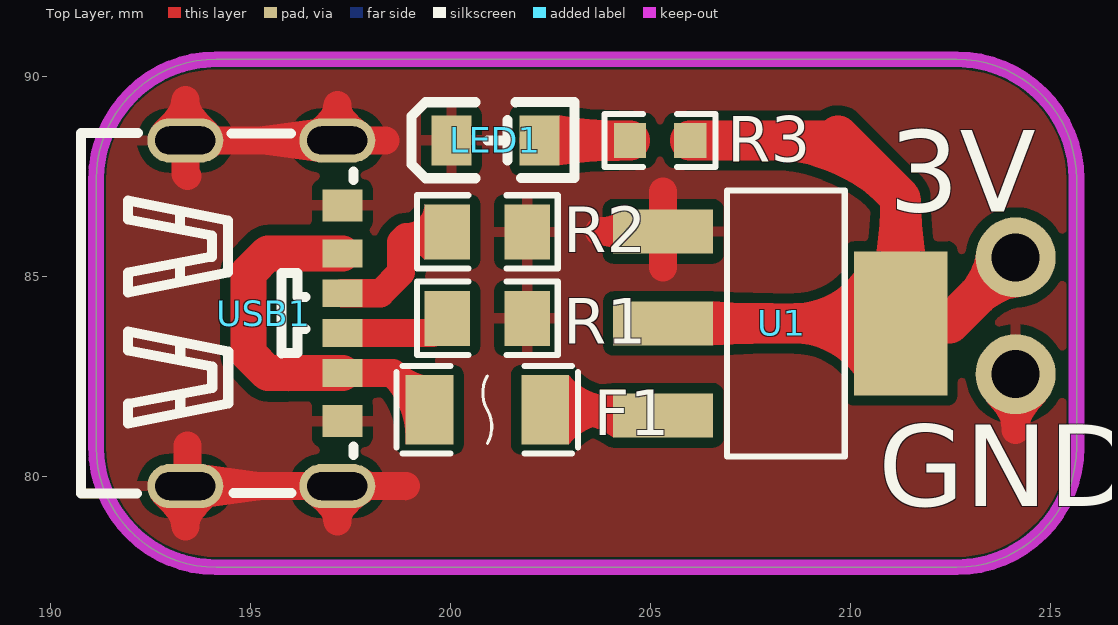
[diagram p0: Top Layer view]
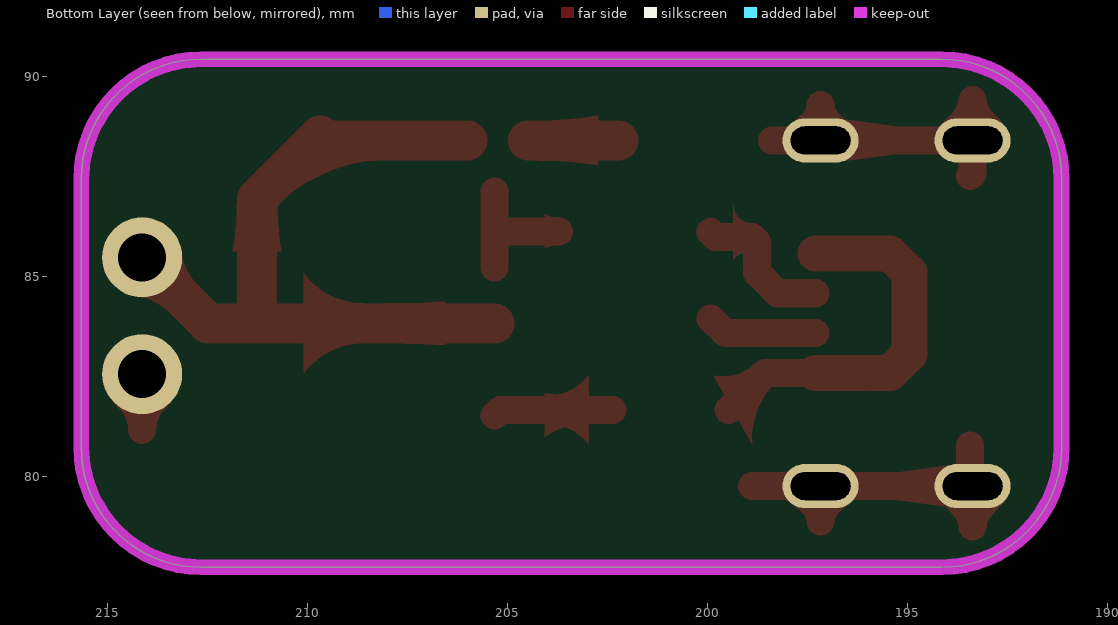
[diagram p1: Bottom Layer view, seen from below]
# Altium PCB MISC49884.pcbdoc
Units mm, origin at the board's own origin, x right, y up, seen from the top; angles counter-clockwise.
Board outline 24.51 x 12.7 mm, 2 copper layers (Top Layer, Bottom Layer), stack 1.58 mm thick; 7 components, 7 nets, 26 pads, 0 vias.

## Layer stack, top to bottom
Top Solder Mask Layer: solder mask 0.01, Dk 3.3
Top Layer: signal copper 0.035
Dielectric1: surface 1.51, FR4, Dk 4.5
Bottom Layer: signal copper 0.035
Bottom Solder Mask Layer: solder mask 0.01, Dk 3.3

## Board outline
194.135,90.424 ccw(c194.135,87.424) 191.135,87.424 191.135,80.724 ccw(c194.135,80.724) 194.135,77.724 212.646,77.724 ccw(c212.646,80.724) 215.646,80.724 215.646,87.424 ccw(c212.646,87.424) 212.646,90.424

## Design rules (kind name [scope] priority, off if disabled: settings)
BoardOutlineClearance copperThickness2oz_1 [All] p2 off: genericclearance=0.203 ignorepadtopadclearanceinfootprint=FALSE except(0: Arc-SplitContinuation Track-SplitContinuation SMDPad-SplitContinuation THPad-SplitContinuation Via-SplitContinuation Fill-SplitContinuation Region-SplitContinuation Poly-SplitContinuation Text-SplitContinuation Hole-SplitContinuation; 0.152: SMDPad-CutoutEdge THPad-CutoutEdge Via-CutoutEdge Fill-CutoutEdge Region-CutoutEdge Text-CutoutEdge Hole-CutoutEdge; 0.254: Poly-OutlineEdge Poly-CutoutEdge; 0.3: Arc-OutlineEdge Track-OutlineEdge SMDPad-OutlineEdge THPad-OutlineEdge Via-OutlineEdge Fill-OutlineEdge Region-OutlineEdge Text-OutlineEdge Hole-OutlineEdge Arc-CutoutEdge Track-CutoutEdge)
BoardOutlineClearance Plane_innerPlane_1 [All] p4 off: genericclearance=0.102 ignorepadtopadclearanceinfootprint=FALSE except(0: Arc-SplitContinuation Track-SplitContinuation SMDPad-SplitContinuation THPad-SplitContinuation Via-SplitContinuation Fill-SplitContinuation Region-SplitContinuation Poly-SplitContinuation Text-SplitContinuation Hole-SplitContinuation; 0.152: SMDPad-CutoutEdge THPad-CutoutEdge Via-CutoutEdge Fill-CutoutEdge Region-CutoutEdge Text-CutoutEdge Hole-CutoutEdge; 0.254: Poly-OutlineEdge Poly-CutoutEdge; 0.3: Arc-OutlineEdge Track-OutlineEdge SMDPad-OutlineEdge THPad-OutlineEdge Via-OutlineEdge Fill-OutlineEdge Region-OutlineEdge Text-OutlineEdge Hole-OutlineEdge Arc-CutoutEdge Track-CutoutEdge)
BoardOutlineClearance Copper_copperRegion_1 [All] p6 off: genericclearance=0.102 ignorepadtopadclearanceinfootprint=FALSE except(0: Arc-SplitContinuation Track-SplitContinuation SMDPad-SplitContinuation THPad-SplitContinuation Via-SplitContinuation Fill-SplitContinuation Region-SplitContinuation Poly-SplitContinuation Text-SplitContinuation Hole-SplitContinuation; 0.152: SMDPad-CutoutEdge THPad-CutoutEdge Via-CutoutEdge Fill-CutoutEdge Region-CutoutEdge Text-CutoutEdge Hole-CutoutEdge; 0.254: Poly-OutlineEdge Poly-CutoutEdge; 0.3: Arc-OutlineEdge Track-OutlineEdge SMDPad-OutlineEdge THPad-OutlineEdge Via-OutlineEdge Fill-OutlineEdge Region-OutlineEdge Text-OutlineEdge Hole-OutlineEdge Arc-CutoutEdge Track-CutoutEdge)
BoardOutlineClearance copperThickness1oz_1 [All] p8: genericclearance=0.102 ignorepadtopadclearanceinfootprint=FALSE except(0: Arc-SplitContinuation Track-SplitContinuation SMDPad-SplitContinuation THPad-SplitContinuation Via-SplitContinuation Fill-SplitContinuation Region-SplitContinuation Poly-SplitContinuation Text-SplitContinuation Hole-SplitContinuation; 0.152: SMDPad-CutoutEdge THPad-CutoutEdge Via-CutoutEdge Fill-CutoutEdge Region-CutoutEdge Text-CutoutEdge Hole-CutoutEdge; 0.254: Poly-OutlineEdge Poly-CutoutEdge; 0.3: Arc-OutlineEdge Track-OutlineEdge SMDPad-OutlineEdge THPad-OutlineEdge Via-OutlineEdge Fill-OutlineEdge Region-OutlineEdge Text-OutlineEdge Hole-OutlineEdge Arc-CutoutEdge Track-CutoutEdge)
Clearance copperThickness2oz [All] p1 off: gap=0.203 ignorepadtopadclearanceinfootprint=FALSE except(0.152: SMDPad-Track SMDPad-SMDPad THPad-Track SMDPad-THPad THPad-THPad Track-Via SMDPad-Via THPad-Via Via-Via Fill-Track Region-Track Fill-SMDPad Region-SMDPad Fill-THPad Region-THPad Fill-Via Region-Via Fill-Fill Fill-Region Region-Region Arc-Track Arc-SMDPad Arc-THPad Arc-Via Fill-Arc Region-Arc Arc-Arc Text-Track SMDPad-Text Text-THPad Text-Via Fill-Text Region-Text Arc-Text Text-Text Hole-Track Hole-SMDPad Hole-THPad Hole-Via Fill-Hole Region-Hole Hole-Arc Hole-Text; 0.254: Poly-Track Poly-SMDPad Poly-THPad Poly-Via Poly-Fill Poly-Region Poly-Poly Poly-Arc Poly-Text Poly-Hole)
Clearance Plane_innerPlane [All] p3 off: gap=0.102 ignorepadtopadclearanceinfootprint=FALSE except(0.152: SMDPad-Track SMDPad-SMDPad THPad-Track SMDPad-THPad THPad-THPad Track-Via SMDPad-Via THPad-Via Via-Via Fill-Track Region-Track Fill-SMDPad Region-SMDPad Fill-THPad Region-THPad Fill-Via Region-Via Fill-Fill Fill-Region Region-Region Arc-Track Arc-SMDPad Arc-THPad Arc-Via Fill-Arc Region-Arc Arc-Arc Text-Track SMDPad-Text Text-THPad Text-Via Fill-Text Region-Text Arc-Text Text-Text Hole-Track Hole-SMDPad Hole-THPad Hole-Via Fill-Hole Region-Hole Hole-Arc Hole-Text; 0.254: Poly-Track Poly-SMDPad Poly-THPad Poly-Via Poly-Fill Poly-Region Poly-Poly Poly-Arc Poly-Text Poly-Hole)
Clearance Copper_copperRegion [All] p5 off: gap=0.102 ignorepadtopadclearanceinfootprint=FALSE except(0.152: SMDPad-Track SMDPad-SMDPad THPad-Track SMDPad-THPad THPad-THPad Track-Via SMDPad-Via THPad-Via Via-Via Fill-Track Region-Track Fill-SMDPad Region-SMDPad Fill-THPad Region-THPad Fill-Via Region-Via Fill-Fill Fill-Region Region-Region Arc-Track Arc-SMDPad Arc-THPad Arc-Via Fill-Arc Region-Arc Arc-Arc Text-Track SMDPad-Text Text-THPad Text-Via Fill-Text Region-Text Arc-Text Text-Text Hole-Track Hole-SMDPad Hole-THPad Hole-Via Fill-Hole Region-Hole Hole-Arc Hole-Text; 0.254: Poly-Track Poly-SMDPad Poly-THPad Poly-Via Poly-Fill Poly-Region Poly-Poly Poly-Arc Poly-Text Poly-Hole)
Clearance copperThickness1oz [All] p7: gap=0.102 ignorepadtopadclearanceinfootprint=FALSE except(0.152: SMDPad-Track SMDPad-SMDPad THPad-Track SMDPad-THPad THPad-THPad Track-Via SMDPad-Via THPad-Via Via-Via Fill-Track Region-Track Fill-SMDPad Region-SMDPad Fill-THPad Region-THPad Fill-Via Region-Via Fill-Fill Fill-Region Region-Region Arc-Track Arc-SMDPad Arc-THPad Arc-Via Fill-Arc Region-Arc Arc-Arc Text-Track SMDPad-Text Text-THPad Text-Via Fill-Text Region-Text Arc-Text Text-Text Hole-Track Hole-SMDPad Hole-THPad Hole-Via Fill-Hole Region-Hole Hole-Arc Hole-Text; 0.254: Poly-Track Poly-SMDPad Poly-THPad Poly-Via Poly-Fill Poly-Region Poly-Poly Poly-Arc Poly-Text Poly-Hole)
DiffPairsRouting differentialPair [All] p1: maxlimit=0.152 minlimit=0.152 mostfreqgap=0.152 toplayer_minwidth=0.127 toplayer_prefwidth=0.254 toplayer_maxwidth=2.54 toplayer_mingap=0.152 toplayer_prefgap=0.152 toplayer_maxgap=0.152 bottomlayer_minwidth=0.127 bottomlayer_prefwidth=0.254 bottomlayer_maxwidth=2.54 bottomlayer_mingap=0.152 bottomlayer_prefgap=0.152 bottomlayer_maxgap=0.152 maxuncoupledlength=0.254
HoleToHoleClearance otherClearance [All] p1: gap=0.3 allowstackedmicrovias=TRUE
Length netLength [All] p1: minlimit=0 maxlimit=0
PasteMaskExpansion pasteMaskExpansion [All] p1: expansion=0
PlaneConnect innerPlane [All] p1: planeconnectstyle=Relief reliefexpansion=0.508 reliefentries=4 reliefconductorwidth=0.254 reliefairgap=0.254
PolygonConnect copperRegion [All] p1: connectstyle=Relief reliefconductorwidth=0.254 reliefentries=4 polygonreliefangle="90 Angle" airgapwidth=0.254 via.connectstyle=Relief via.reliefconductorwidth=0.254 via.reliefentries=4 via.polygonreliefangle="90 Angle" via.airgapwidth=0.254
RoutingVias viaSize [All] p1: holewidth=0.305 width=0.61 viastyle="Through Hole" minholewidth=0.3 minwidth=0.5 maxholewidth=6.3 maxwidth=10
SolderMaskExpansion solderMaskExpansion [IsVia] p1: expansion=-25.4 istentingtop=TRUE
SolderMaskExpansion solderMaskExpansion [All] p2: expansion=0.051 istentingtop=FALSE
Width copperThickness2oz_2 [All] p1 off: maxlimit=2.54 minlimit=0.203 preferedwidth=0.254
Width copperThickness1oz_2 [All] p2: maxlimit=2.54 minlimit=0.127 preferedwidth=0.254

## Components (designator, comment, footprint, x,y, rotation, side; value= is the part's Value field where it differs from the comment)
F1 "BSMD1206-200-6V" F1206 200.914,81.661 r180 top
LED1 "" LED_0805 201.168,88.392 r0 top
R1 "5.1k" R0805 200.914,83.947 r0 top
R2 "5.1k" R0805 200.914,86.106 r0 top
R3 "1K" R0603 205.232,88.392 r180 top
U1 "AMS1117-3.3" SOT-223-3_L6.5-W3.4-P2.30-LS7.0-BR 208.28,83.82 r180 top
USB1 "TYPE_C_SMD_6P" TYPE-C-SMD_TYPE-C-6P 195.326,84.074 r270 top

## Footprints (in the part's own frame and the unit in brackets; to place one, negate y for a bottom-side part, rotate by r counter-clockwise, add the part's x,y. Pads: shape width x height; smd on the part's side, far side on the other; paste and mask are expansions set on the pad)
F1206 [mm]
  rect 1.19x1.728 smd: 1(-1.445,0) 2(1.445,0)
  silkscreen extent -2.27,-1.09 2.27,1.09
LED_0805 [mm]
  rect 1x1.25 smd paste+0 mask+0.051: 1(-1.15,0.005) 2(1.05,0.005)
  silkscreen extent -2.15,-0.94 1.93,0.97
R0603 [mm]
  rect 0.806x0.864 smd paste-100 mask+0.051: 1(-0.753,0) 2(0.753,0)
  silkscreen extent -1.39,-0.66 1.39,0.66
R0805 [mm]
  rect 1.133x1.377 smd paste-100 mask+0.051: 1(-1,0) 2(1,0)
  silkscreen extent -1.76,-0.92 1.76,0.92
SOT-223-3_L6.5-W3.4-P2.30-LS7.0-BR [mm]
  rect 2.5x1.1 smd: 1(2.97,-2.3) 2(2.97,0) 3(2.97,2.3)
  rect 2.34x3.6 smd: 4(-2.97,0)
  silkscreen extent -1.57,-3.33 1.37,3.33
TYPE-C-SMD_TYPE-C-6P [mm]
  oval 1.1x1.9 hole 0.7 slot 1.5 at 90 deg: 7(-4.32,-1.963) 7(-4.32,1.838) 7(4.32,-1.963) 7(4.32,1.838)
  rect 0.7x1 smd paste-100 mask+0.051: A5(-0.5,1.963) A9(1.5,1.963) B5(0.5,1.963) B9(-1.5,1.963)
  rect 0.8x1 smd paste-100 mask+0.051: A12(2.7,1.963) B12(-2.7,1.963)
  silkscreen extent -4.5,-4.56 4.5,2.24

## Free pads (board coordinates)
  round 2 hole 1.2: 1(214.122,82.55) 1(214.122,85.471)

## Nets (pads, with @x,y where several pads share a name; then routed paths per layer and width w, separated by ;. In a path a pad name is that pad's centre, name@x,y a point inside that pad or via, vN(x,y) a via of type N, cw(c..) or ccw(c..) an arc to the next point about the centre after c; other vN are vias at no path point)
3.3V: pad.1@214.122,85.471 R3.1 U1.2 U1.4 | length 18.6
  Top Layer w1: U1.2 U1.4 ; R3.1 209.55,88.392 209.677,88.519 211.25,86.946 U1.4 ; pad.1@214.122,85.471 212.471,83.82 U1.4
$1N166: R1.1 USB1.B5 | length 2.8
  Top Layer w0.7: USB1.B5 199.541,83.574 R1.1
$1N167: R2.1 USB1.A5 | length 3.7
  Top Layer w0.7: USB1.A5 198.239,84.574 198.755,85.09 198.755,85.852 198.882,85.979 199.787,85.979 R2.1
$1N428: LED1.2 R3.2 | length 2.3
  Top Layer w1: LED1.2 202.223,88.392 R3.2
$1N1208: F1.2 USB1.A9 USB1.B9 | length 9.7
  Top Layer w0.7: USB1.A9 198.556,82.574 F1.2
  Top Layer w0.9: USB1.A9 195.429,82.574 194.945,83.058 194.945,85.09 195.429,85.574 USB1.B9
+5V: F1.1 U1.3 | length 3
  Top Layer w0.7: F1.1 205.169,81.661 U1.3
GND: LED1.1 pad.1@214.122,82.55 R1.2 R2.2 U1.1 USB1.7 USB1.A12 USB1.B12 | length 21.2
  Top Layer w0.7: 193.363,78.74 USB1.7@193.363,79.754 ; 193.363,89.408 USB1.7@193.363,88.394 ; 193.421,80.772 193.421,79.812 USB1.7@193.363,79.754 ; 193.421,87.503 193.363,87.561 USB1.7@193.363,88.394 ; 197.164,78.867 USB1.7@197.164,79.754 ; 197.164,89.281 USB1.7@197.164,88.394 ; 198.374,88.394 USB1.7@197.164,88.394 ; 198.882,79.754 USB1.7@197.164,79.754 ; 203.708,86.12 U1.1 ; 205.31,85.217 U1.1 ; 205.31,87.122 U1.1 ; 214.122,81.153 pad.1@214.122,82.55 ; USB1.7@193.363,79.754 USB1.7@197.164,79.754 ; USB1.7@193.363,88.394 USB1.7@197.164,88.394

## Polygon pours and split planes (outlines as drawn)
GND on Top Layer (solid, remove dead copper, pour order 4): 189.738,92.456 189.738,76.2 216.281,76.2 216.281,92.456
GND on Top Layer (solid, remove dead copper, pour order 0): 149.733,161.544 149.733,123.444 187.325,123.444 187.325,161.544
GND on Bottom Layer (solid, remove dead copper, pour order 6): 76.2,136.144 76.2,94.869 115.824,94.869 115.824,136.144

## Keep-outs
Board Outline Layer:
  the board outline again, w0.399

## Other copper
Top Layer:
  region net 3.3V: 208.58,84.32 208.58,83.32 208.773,83.31 208.964,83.28 209.15,83.231 209.331,83.163 209.504,83.077 209.667,82.973 209.818,82.853 209.956,82.718 210.08,82.57 210.08,85.07 209.956,84.922 209.818,84.787 209.667,84.667 209.504,84.563 209.331,84.477 209.15,84.409 208.964,84.36 208.773,84.33 208.58,84.32
  region net 3.3V: 208.06,83.32 208.06,84.32 207.56,84.326 207.06,84.342 206.56,84.37 206.56,83.27 207.06,83.298 207.56,83.314 208.06,83.32
  region net 3.3V: 211.75,86.946 210.75,86.946 210.743,86.613 210.724,86.281 210.691,85.95 210.645,85.62 211.855,85.62 211.809,85.95 211.776,86.281 211.757,86.613 211.75,86.946
  region net 3.3V: 208.304,87.892 208.382,87.89 208.48,87.882 208.601,87.866 208.745,87.839 208.933,87.794 209.146,87.73 209.381,87.645 209.613,87.548 209.837,87.44 210.031,87.333 210.178,87.242 210.297,87.159 210.393,87.085 210.466,87.021 210.511,86.978 211.218,87.685 210.158,88.038 208.304,88.892
  region net $1N428: 204.218,87.892 204.218,88.892 203.841,88.9 203.465,88.925 203.091,88.965 202.718,89.022 202.718,87.772 203.091,87.825 203.466,87.862 203.842,87.884 204.218,87.892
  region net $1N167: 198.882,86.329 198.882,85.629 198.987,85.62 199.089,85.593 199.185,85.55 199.272,85.491 199.348,85.417 199.348,86.795 199.339,86.704 199.312,86.616 199.269,86.536 199.211,86.465 199.141,86.407 199.06,86.364 198.973,86.338
  region net $1N1208: 198.556,82.224 197.739,82.574 195.939,82.124 195.939,83.024 196.839,82.574 198.556,82.924
  region net $1N1208: 198.803,82.821 198.309,82.327 198.434,82.188 198.546,82.039 198.643,81.879 198.724,81.711 198.789,81.535 198.837,81.355 198.867,81.17 198.879,80.984 198.874,80.797 199.842,82.525 199.703,82.502 199.563,82.496 199.422,82.509 199.285,82.539 199.152,82.586 199.026,82.649 198.909,82.728 198.803,82.821
  region net +5V: 204.004,81.311 204.004,82.011 203.853,82.02 203.704,82.045 203.559,82.087 203.42,82.146 203.288,82.219 203.166,82.307 203.054,82.409 202.954,82.522 202.954,80.8 203.054,80.913 203.166,81.015 203.288,81.103 203.42,81.176 203.559,81.235 203.704,81.277 203.853,81.302 204.004,81.311
  region net +5V: 203.01,82.011 203.01,81.311 203.197,81.301 203.381,81.272 203.562,81.224 203.737,81.157 203.903,81.072 204.06,80.97 204.06,82.07 203.711,82.037 203.361,82.018 203.01,82.011
  region net 3.3V: 212.806,84.862 213.513,84.155 213.542,84.182 213.593,84.224 213.651,84.265 213.713,84.304 213.78,84.341 213.849,84.375 213.92,84.405 213.99,84.431 214.058,84.451 214.102,84.462 214.144,84.469 214.185,84.473 213.124,85.534 213.12,85.493 213.113,85.451 213.102,85.407 213.082,85.339 213.056,85.269 213.026,85.198 212.992,85.129 212.955,85.062 212.916,85 212.875,84.942 212.833,84.891
  region net GND: 203.708,86.47 203.708,85.77 203.828,85.762 203.946,85.737 204.06,85.696 204.06,86.544 203.946,86.503 203.828,86.478
  region net GND: 213.772,81.189 214.472,81.189 214.473,81.23 214.477,81.27 214.483,81.309 214.492,81.346 214.502,81.382 214.515,81.417 214.53,81.45 214.546,81.483 214.57,81.526 214.597,81.567 214.634,81.617 214.691,81.687 214.872,81.889 213.372,81.889 213.562,81.677 213.618,81.607 213.654,81.557 213.68,81.515 213.704,81.472 213.72,81.439 213.733,81.405 213.745,81.37 213.755,81.334 213.763,81.296 213.768,81.257 213.771,81.217
  region net GND: 196.814,78.867 197.514,78.867 197.515,78.891 197.518,78.914 197.523,78.937 197.531,78.959 197.54,78.98 197.551,79.001 197.563,79.021 197.577,79.041 197.609,79.079 197.645,79.115 197.706,79.168 197.88,79.306 197.941,79.359 197.978,79.397 198.011,79.436 198.026,79.456 198.039,79.477 196.289,79.477 196.302,79.456 196.316,79.436 196.349,79.397 196.386,79.359 196.447,79.306 196.622,79.168 196.682,79.115 196.718,79.079 196.75,79.041 196.764,79.021 196.776,79.001 196.787,78.98 196.796,78.959 196.804,78.937 196.809,78.914 196.812,78.891
  region net GND: 198.882,79.404 198.882,80.104 198.802,80.102 198.71,80.094 198.593,80.076 198.401,80.042 198.347,80.035 198.306,80.032 198.267,80.031 198.24,80.032 198.213,80.035 198.187,80.039 198.16,80.045 198.133,80.052 198.105,80.062 198.078,80.073 198.049,80.087 198.02,80.103 197.976,80.131 197.93,80.165 197.914,80.178 197.914,79.33 197.961,79.367 198.006,79.397 198.035,79.414 198.063,79.429 198.091,79.441 198.119,79.451 198.146,79.46 198.173,79.467 198.2,79.471 198.227,79.475 198.253,79.477 198.293,79.477 198.333,79.475 198.388,79.469 198.562,79.438 198.693,79.417 198.783,79.408 198.862,79.404
  region net GND: 195.238,79.404 195.238,80.104 193.784,80.302 193.763,80.304 193.763,79.204 195.217,79.402
  region net GND: 193.013,78.74 193.713,78.74 193.715,78.764 193.718,78.789 193.723,78.813 193.731,78.837 193.74,78.861 193.751,78.885 193.777,78.933 193.809,78.981 193.845,79.028 193.905,79.099 194.101,79.303 194.16,79.37 194.195,79.413 194.225,79.456 194.238,79.477 192.488,79.477 192.516,79.434 192.549,79.391 192.605,79.326 192.8,79.122 192.863,79.052 192.901,79.005 192.935,78.957 192.964,78.909 192.976,78.885 192.987,78.861 192.996,78.837 193.004,78.813 193.009,78.789 193.012,78.764
  region net GND: 195.238,88.044 195.238,88.744 195.144,88.741 195.057,88.734 194.957,88.719 194.727,88.674 194.631,88.657 194.585,88.652 194.539,88.649 194.508,88.65 194.478,88.651 194.447,88.655 194.416,88.66 194.385,88.667 194.353,88.677 194.321,88.689 194.289,88.703 194.256,88.72 194.221,88.74 194.169,88.775 194.114,88.818 194.114,87.97 194.169,88.013 194.221,88.048 194.256,88.068 194.289,88.085 194.321,88.099 194.353,88.111 194.385,88.121 194.416,88.128 194.447,88.133 194.478,88.137 194.508,88.138 194.554,88.138 194.6,88.134 194.663,88.126 194.864,88.086 194.996,88.062 195.1,88.05 195.19,88.045
  region net GND: 195.289,88.744 195.289,88.044 196.764,87.844 196.764,88.944
  region net GND: 197.514,89.281 196.814,89.281 196.812,89.257 196.809,89.234 196.804,89.211 196.796,89.189 196.787,89.168 196.776,89.147 196.764,89.127 196.75,89.107 196.718,89.069 196.682,89.033 196.622,88.98 196.447,88.842 196.386,88.789 196.349,88.751 196.316,88.712 196.302,88.692 196.289,88.671 198.039,88.671 198.026,88.692 198.011,88.712 197.978,88.751 197.941,88.789 197.88,88.842 197.706,88.98 197.645,89.033 197.609,89.069 197.577,89.107 197.563,89.127 197.551,89.147 197.54,89.168 197.531,89.189 197.523,89.211 197.518,89.234 197.515,89.257
  region net GND: 193.713,89.408 193.013,89.408 193.012,89.384 193.009,89.359 193.004,89.335 192.996,89.311 192.987,89.287 192.976,89.263 192.95,89.215 192.918,89.167 192.882,89.12 192.822,89.049 192.626,88.845 192.567,88.778 192.532,88.735 192.502,88.692 192.488,88.671 194.238,88.671 194.211,88.714 194.178,88.757 194.122,88.822 193.927,89.026 193.864,89.096 193.826,89.143 193.792,89.191 193.763,89.239 193.751,89.263 193.74,89.287 193.731,89.311 193.723,89.335 193.718,89.359 193.715,89.384

## Silkscreen, mask and mechanical layers (free items; w line width, h text height)
Top Silkscreen Layer:
  text "3V" at 210.947,86.614 h2.03
  text "GND" at 210.693,79.248 h2.03